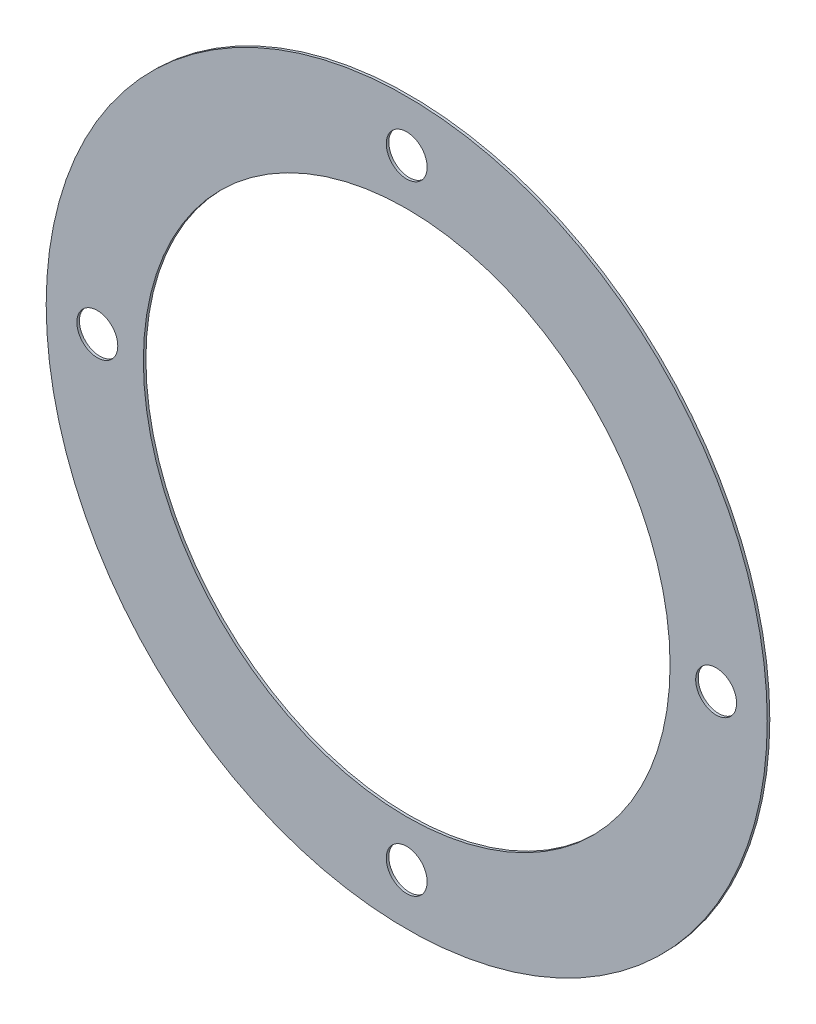
SolidWorks part; units mm, degrees
ref_plane "Front Plane" through (0, 0, 0) normal (0, 0, 1) x (1, 0, 0)
ref_plane "Top Plane" through (0, 0, 0) normal (0, 1, 0) x (1, 0, 0)
ref_plane "Right Plane" through (0, 0, 0) normal (1, 0, 0) x (0, 0, -1)
sketch "Sketch1" plane through (0, 0, 0) normal (0, 0, 1) x (1, 0, 0)
  circle A0 centre (0, 0) radius 51.5
  circle A1 centre (0, 0) radius 70.5
  dimension "D1" = 141
  dimension "D2" = 103
extrude "Boss-Extrude1" add sketch "Sketch1" along normal blind 0.5
sketch "Sketch2" plane through (0, 0, 0.5) normal (0, 0, 1) x (1, 0, 0)
  circle A1 centre (0, -60.5) radius 4
  circle A2 centre (-60.5, 0) radius 4
  circle A3 centre (0, 60.5) radius 4
  circle A4 centre (60.5, 0) radius 4
  point P14 (0, 0)
  dimension "D2" = 8
  dimension "D3" = 4
extrude "Cut-Extrude1" cut sketch "Sketch2" against normal blind 0.5
